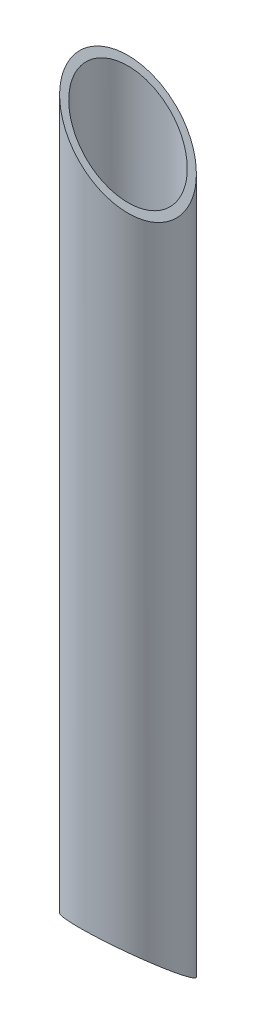
from build123d import *

# Parameters (mm, degrees)
SKETCH1_R               = 30
SKETCH1_R_2             = 26
BOSS_EXTRUDE1_DEPTH     = 490
CUT_EXTRUDE1_DEPTH      = 492.833305094
CUT_EXTRUDE1_DEPTH_BACK = 492.833305094
CUT_EXTRUDE2_DEPTH      = 492.833305094
CUT_EXTRUDE2_DEPTH_BACK = 492.833305094


with BuildPart() as part:
    # Sketch1 → Boss-Extrude1 (new body)
    with BuildSketch(Plane(origin=(0, 0, 0), x_dir=(1, 0, 0), z_dir=(0, 1, 0))):
        with Locations(Location((0, 0, 0), (0, 0, 270))):
            Circle(SKETCH1_R)
        with Locations(Location((0, 0, 0), (0, 0, 270))):
            Circle(SKETCH1_R_2, mode=Mode.SUBTRACT)
    extrude(amount=BOSS_EXTRUDE1_DEPTH)

    # Sketch2 → Cut-Extrude1 (cut, two sides: drawn at the far end of the back side and taken through both)
    with BuildSketch(Plane.XY.offset(-CUT_EXTRUDE1_DEPTH_BACK)):
        Polygon((-735.21145484, 1195.21145484), (-30, 490), (243.212319076, 216.787680924), (948.423773916, -488.423773916), (2358.846683596, 921.999135764), (675.21145484, 2605.63436452), align=None)
    extrude(amount=CUT_EXTRUDE1_DEPTH + CUT_EXTRUDE1_DEPTH_BACK, mode=Mode.SUBTRACT)

    # Sketch3 → Cut-Extrude2 (cut, two sides: drawn at the far end of the back side and taken through both)
    with BuildSketch(Plane(origin=(0, 0, 0), x_dir=(0, 0, -1), z_dir=(1, 0, 0)).offset(-CUT_EXTRUDE2_DEPTH_BACK)):
        Polygon((805.062902356, -627.63356305), (30, 0), (-69.882630866, 80.883359669), (-844.945533223, 708.516922719), (-2100.212659322, -841.608881993), (-450.204223743, -2177.759367762), align=None)
    extrude(amount=CUT_EXTRUDE2_DEPTH + CUT_EXTRUDE2_DEPTH_BACK, mode=Mode.SUBTRACT)


solid = part.part
